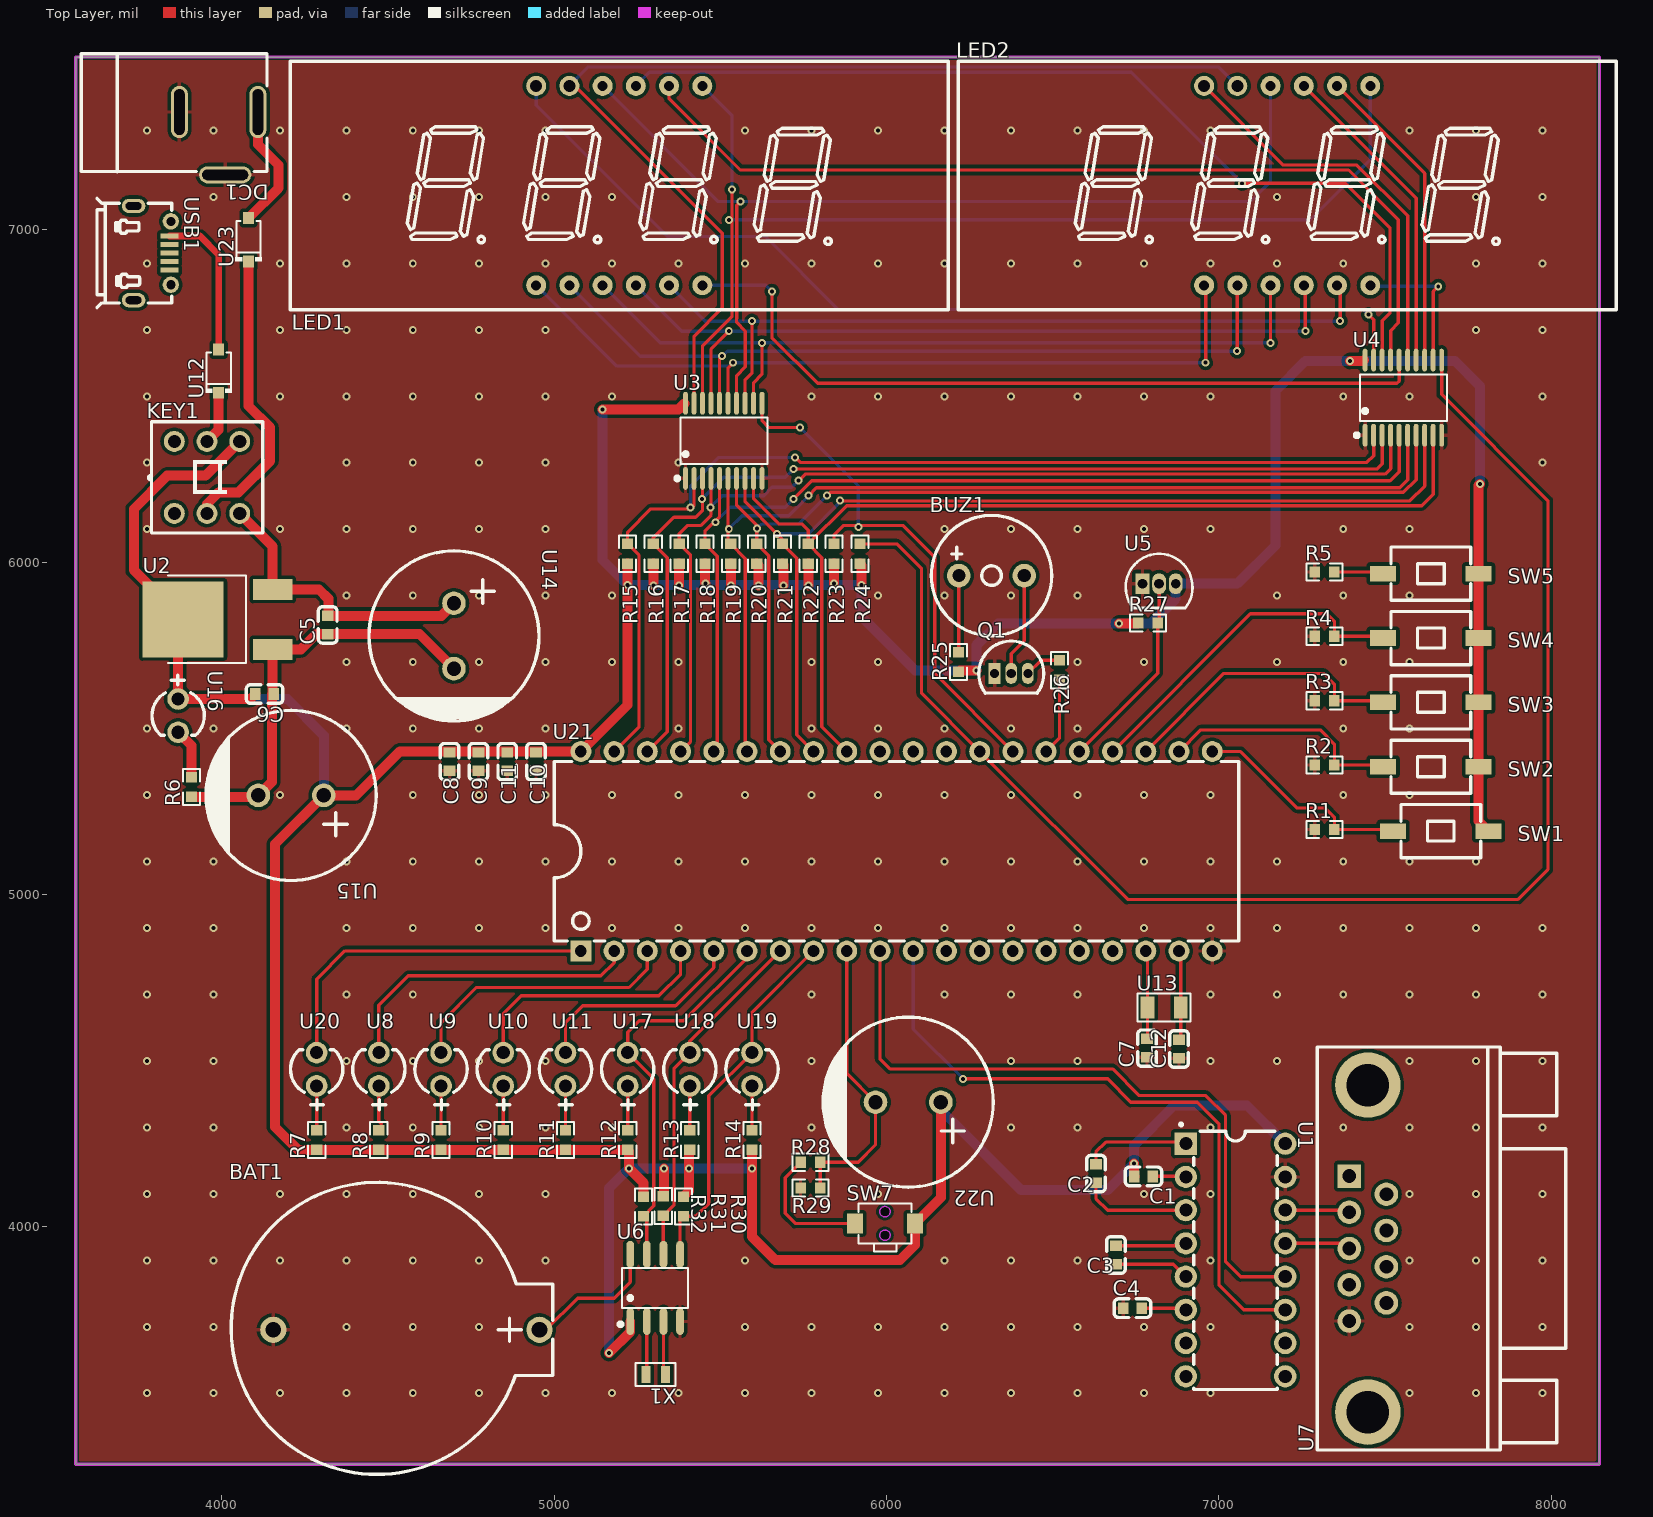
[diagram p0: Top Layer view]
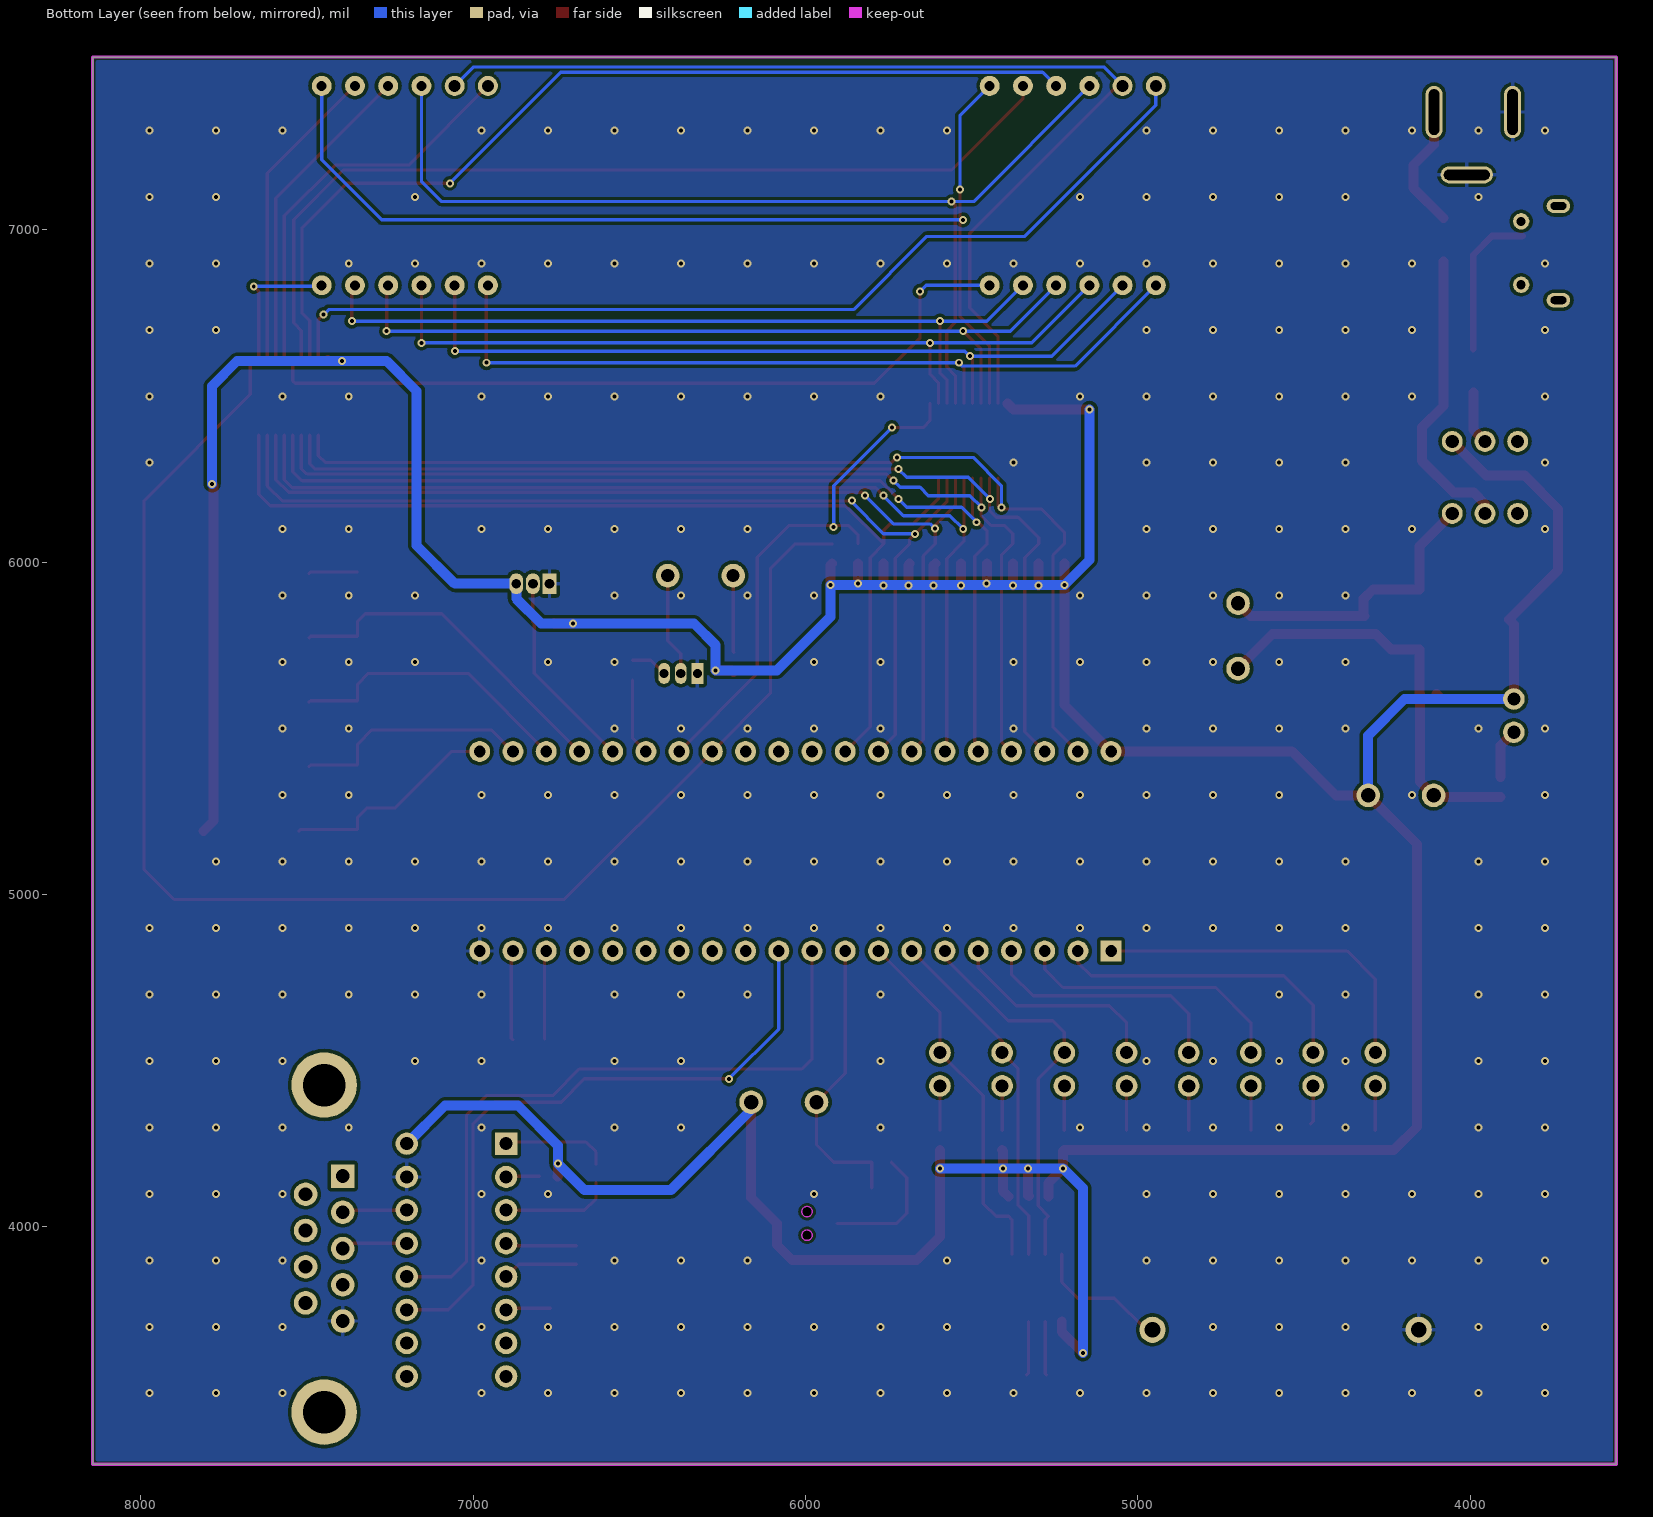
[diagram p1: Bottom Layer view, seen from below]
# Altium PCB MISC51895.pcbdoc
Units mil, origin at the board's own origin, x right, y up, seen from the top; angles counter-clockwise.
Board outline 4585 x 4235 mil, 2 copper layers (Top Layer, Bottom Layer), stack 62.206 mil thick; 82 components, 78 nets, 302 pads, 351 vias.

## Layer stack, top to bottom
Top Solder Mask Layer: solder mask 0.394, Dk 3.3
Top Layer: signal copper 1.379
Dielectric1: surface 59.449, FR4, Dk 4.5
Bottom Layer: signal copper 1.378
Bottom Solder Mask Layer: solder mask 0.394, Dk 3.3

## Board outline
3560,7520 3560,3285 8145,3285 8145,7520

## Design rules (kind name [scope] priority, off if disabled: settings)
BoardOutlineClearance copperThickness2oz_1 [All] p2 off: genericclearance=7.99 ignorepadtopadclearanceinfootprint=FALSE except(0: Arc-SplitContinuation Track-SplitContinuation SMDPad-SplitContinuation THPad-SplitContinuation Via-SplitContinuation Fill-SplitContinuation Region-SplitContinuation Poly-SplitContinuation Text-SplitContinuation Hole-SplitContinuation; 5.98: Arc-CutoutEdge SMDPad-CutoutEdge THPad-CutoutEdge Via-CutoutEdge Fill-CutoutEdge Region-CutoutEdge Text-CutoutEdge; 6.93: Hole-OutlineEdge Hole-CutoutEdge; 10: Poly-OutlineEdge Poly-CutoutEdge; 11.81: Arc-OutlineEdge Track-OutlineEdge SMDPad-OutlineEdge THPad-OutlineEdge Via-OutlineEdge Fill-OutlineEdge Region-OutlineEdge Text-OutlineEdge Track-CutoutEdge)
BoardOutlineClearance copperThickness1oz_1 [All] p4: genericclearance=4.02 ignorepadtopadclearanceinfootprint=FALSE except(0: Arc-SplitContinuation Track-SplitContinuation SMDPad-SplitContinuation THPad-SplitContinuation Via-SplitContinuation Fill-SplitContinuation Region-SplitContinuation Poly-SplitContinuation Text-SplitContinuation Hole-SplitContinuation; 6: SMDPad-CutoutEdge THPad-CutoutEdge Via-CutoutEdge Fill-CutoutEdge Region-CutoutEdge Text-CutoutEdge; 6.93: Hole-OutlineEdge Hole-CutoutEdge; 10: Poly-OutlineEdge Poly-CutoutEdge; 11.8: Arc-OutlineEdge Track-OutlineEdge SMDPad-OutlineEdge THPad-OutlineEdge Via-OutlineEdge Fill-OutlineEdge Region-OutlineEdge Text-OutlineEdge; 11.81: Arc-CutoutEdge Track-CutoutEdge)
Clearance copperThickness2oz [All] p1 off: gap=7.99 ignorepadtopadclearanceinfootprint=FALSE except(5.98: SMDPad-Track SMDPad-SMDPad THPad-Track SMDPad-THPad THPad-THPad Track-Via SMDPad-Via THPad-Via Via-Via Fill-Track Region-Track Fill-SMDPad Region-SMDPad Fill-THPad Region-THPad Fill-Via Region-Via Fill-Fill Fill-Region Region-Region Arc-Track Arc-SMDPad Arc-THPad Arc-Via Fill-Arc Region-Arc Arc-Arc Text-Track SMDPad-Text Text-THPad Text-Via Fill-Text Region-Text Arc-Text Text-Text; 6.93: Hole-Track Hole-SMDPad Hole-THPad Hole-Via Fill-Hole Region-Hole Hole-Arc Hole-Text; 10: Poly-Track Poly-SMDPad Poly-THPad Poly-Via Poly-Fill Poly-Region Poly-Poly Poly-Arc Poly-Text Poly-Hole)
Clearance copperThickness1oz [All] p3: gap=4.02 ignorepadtopadclearanceinfootprint=FALSE except(5.98: SMDPad-Track SMDPad-SMDPad THPad-Track SMDPad-THPad THPad-THPad Track-Via SMDPad-Via THPad-Via Via-Via Fill-Track Region-Track Fill-SMDPad Region-SMDPad Fill-THPad Region-THPad Fill-Via Region-Via Fill-Fill Fill-Region Region-Region; 6: Arc-Track Arc-SMDPad Arc-THPad Arc-Via Fill-Arc Region-Arc Arc-Arc Text-Track SMDPad-Text Text-THPad Text-Via Fill-Text Region-Text Arc-Text Text-Text; 6.93: Hole-Track Hole-SMDPad Hole-THPad Hole-Via Fill-Hole Region-Hole Hole-Arc Hole-Text; 10: Poly-Track Poly-SMDPad Poly-THPad Poly-Via Poly-Fill Poly-Region Poly-Poly Poly-Arc Poly-Text Poly-Hole)
DiffPairsRouting differentialPair [All] p1: maxlimit=6 minlimit=6 mostfreqgap=6 toplayer_minwidth=5 toplayer_prefwidth=10 toplayer_maxwidth=100 toplayer_mingap=6 toplayer_prefgap=6 toplayer_maxgap=6 bottomlayer_minwidth=5 bottomlayer_prefwidth=10 bottomlayer_maxwidth=100 bottomlayer_mingap=6 bottomlayer_prefgap=6 bottomlayer_maxgap=6 maxuncoupledlength=10
HoleToHoleClearance otherClearance [All] p1: gap=11.81 allowstackedmicrovias=TRUE
Length netLength [All] p1: minlimit=0 maxlimit=0
MatchedLengths netLengthTolerance [All] p1: tolerance=1000
PasteMaskExpansion pasteMaskExpansion [All] p1: expansion=0
PlaneConnect innerPlane [All] p1: planeconnectstyle=Relief reliefexpansion=20 reliefentries=4 reliefconductorwidth=10 reliefairgap=10
PolygonConnect copperRegion [(InNet('GND'))] p1: connectstyle=Relief reliefconductorwidth=10 reliefentries=4 polygonreliefangle="90 Angle" airgapwidth=10 via.connectstyle=Relief via.reliefconductorwidth=10 via.reliefentries=4 via.polygonreliefangle="90 Angle" via.airgapwidth=10
RoutingVias viaSize [All] p1: holewidth=12.01 width=24.02 viastyle="Through Hole" minholewidth=11.81 minwidth=19.68 maxholewidth=248.03 maxwidth=393.7
SolderMaskExpansion solderMaskExpansion [IsVia] p1: expansion=-1000 istentingtop=TRUE
SolderMaskExpansion solderMaskExpansion [All] p2: expansion=2 istentingtop=FALSE
Width copperThickness2oz_2 [All] p1 off: maxlimit=100 minlimit=8 preferedwidth=10
Width copperThickness1oz_2 [All] p2: maxlimit=100 minlimit=5 preferedwidth=10

## Components (designator, comment, footprint, x,y, rotation, side; value= is the part's Value field where it differs from the comment)
BAT1 "CR2032-2-1" BAT-TH_CR2032-2-1 4555,3690 r0 top
BUZ1 "Buzzer" BUZ-TH_BD9.0-P5.00-D0.6-FD 6315.73,5959.5 r0 top
C1 "104" C0603 6772.91,4151.65 r180 top
C2 "4.7uF" C0603 6630,4160 r90 top
C3 "4.7uF" C0603 6690,3915 r90 top
C4 "4.7uF" C0603 6740,3755 r0 top
C5 "4.7uF" C0603 4318.1,5811.04 r90 top
C6 "4.7uF" C0603 4128.22,5603.04 r180 top
C7 "100nF" C0603 6783.76,4537.58 r90 top
C8 "4.7uF" C0603 4685,5399.61 r90 top
C9 "4.7uF" C0603 4771.67,5399.61 r90 top
C10 "4.7uF" C0603 4945,5399.61 r90 top
C11 "4.7uF" C0603 4858.33,5399.61 r90 top
C12 "100nF" C0603 6880,4535 r90 top
DC1 "" DC-2.0 3985,7365 r180 top
KEY1 "Non-latching switch 8.5×8.5 silent" SW-TH_6P-L8.5-W8.5-P2.54 3955,6255 r0 top
LED1 "FJ5461AB" LED-SEG-TH_12P-L50.4-W19.0-P2.54-S15.24-BL 5195.44,7133.14 r0 top
LED2 "FJ5461AB" LED-SEG-TH_12P-L50.4-W19.0-P2.54-S15.24-BL 7205.45,7133.14 r0 top
Q1 "2SC945" TO-92-3_L4.9-W3.7-P1.27-L 6375,5665 r0 top
R1 "48.7Ω" R0603 7317.91,5195.61 r0 top
R2 "48.7Ω" R0603 7317.91,5389.3 r0 top
R3 "48.7Ω" R0603 7317.91,5583 r0 top
R4 "48.7Ω" R0603 7317.91,5776.69 r0 top
R5 "48.7Ω" R0603 7317.91,5970.38 r0 top
R6 "10K" R0603 3908.1,5323.04 r90 top
R7 "10K" R0603 4284.92,4261.14 r90 top
R8 "10K" R0603 4472.09,4261.14 r90 top
R9 "10K" R0603 4659.25,4261.14 r90 top
R10 "10K" R0603 4846.42,4261.14 r90 top
R11 "10K" R0603 5033.58,4261.14 r90 top
R12 "10K" R0603 5220.75,4261.14 r90 top
R13 "10K" R0603 5407.91,4261.14 r90 top
R14 "10K" R0603 5595.08,4261.14 r90 top
R15 "10K" R0603 5220.35,6025 r90 top
R16 "10K" R0603 5298.05,6025 r90 top
R17 "10K" R0603 5375.75,6025 r90 top
R18 "10K" R0603 5453.45,6025 r90 top
R19 "10K" R0603 5531.15,6025 r90 top
R20 "10K" R0603 5608.85,6025 r90 top
R21 "10K" R0603 5686.55,6025 r90 top
R22 "10K" R0603 5764.25,6025 r90 top
R23 "10K" R0603 5841.95,6025 r90 top
R24 "10K" R0603 5919.65,6025 r90 top
R25 "50" R0603 6216.06,5699.16 r90 top
R26 "1K" R0603 6520,5675 r90 top
R27 "10K" R0603 6786.25,5816.95 r0 top
R28 "10K" R0603 5770.79,4194.3 r180 top
R29 "10K" R0603 5770.79,4116.6 r0 top
R30 "4.7K" R0603 5388.55,4061.02 r270 top
R31 "4.7K" R0603 5327.76,4062.64 r270 top
R32 "4.7K" R0603 5268.55,4061.02 r270 top
SW1 "SW_PB_ESW_1" KEY-SMD_L6.1-W3.8-LS8.0 7667.63,5190.61 r0 top
SW2 "SW_PB_ESW_1" KEY-SMD_L6.1-W3.8-LS8.0 7637.63,5384.3 r0 top
SW3 "SW_PB_ESW_1" KEY-SMD_L6.1-W3.8-LS8.0 7637.63,5578 r0 top
SW4 "SW_PB_ESW_1" KEY-SMD_L6.1-W3.8-LS8.0 7637.63,5771.69 r0 top
SW5 "SW_PB_ESW_1" KEY-SMD_L6.1-W3.8-LS8.0 7637.63,5965.38 r0 top
SW7 "YD-3410" SW-SMD_L3.9-W2.9-LS4.8-EH-A 5995,4010 r0 top
U1 "MAX232AEJE" PDIP-16_L19.3-W6.5-P2.54-LS7.6-BL 7050,3900 r270 top
U2 "LM1117IDT-5.0" TO-252-2_L6.6-W6.1-P4.57-LS9.7-BR-CW 4017.9,5827.5 r0 top
U3 "74HC573PW/AU118" TSSOP-20_L6.5-W4.4-P0.65-LS6.4-BL 5510,6365 r0 top
U4 "74HC573PW/AU118" TSSOP-20_L6.5-W4.4-P0.65-LS6.4-BL 7555,6495 r0 top
U5 "DS18B20+T&R-HX" TO-92-3_L5.1-W4.1-P1.27-L-1 6820,5935 r0 top
U6 "DS1302Z+T&R-TUDI" SOIC-8_L4.9-W3.9-P1.27-LS6.0-BL 5303.55,3816.02 r0 top
U7 "DB9F" DB9-TH_DB9F_C9900018961 7448.11,3934.4 r90 top
U8 "LED" LED-TH_BD4.0-P2.54-FD_RED 4472.09,4473.89 r90 top
U9 "LED" LED-TH_BD4.0-P2.54-FD_RED 4659.25,4473.89 r90 top
U10 "LED" LED-TH_BD4.0-P2.54-FD_RED 4846.42,4473.89 r90 top
U11 "LED" LED-TH_BD4.0-P2.54-FD_RED 5033.58,4473.89 r90 top
U12 "IN5819" SOD-123_L2.7-W1.7-LS3.8-RD 3990,6575 r90 top
U13 "2.768KHz" CRYSTAL-SMD_L3.2-W1.5-1 6835,4660 r0 top
U14 "CE63V1000uF13*25" CAP-TH_BD13.0-P5.00-D0.6-FD 4698.1,5778.04 r270 top
U15 "10uF" CAP-TH_BD13.0-P5.00-D0.6-FD 4208.1,5298.04 r180 top
U16 "LED" LED-TH_BD4.0-P2.54-FD_RED 3868.1,5538.04 r270 top
U17 "LED" LED-TH_BD4.0-P2.54-FD_RED 5220.75,4473.89 r90 top
U18 "LED" LED-TH_BD4.0-P2.54-FD_RED 5407.91,4473.89 r90 top
U19 "LED" LED-TH_BD4.0-P2.54-FD_RED 5595.08,4473.89 r90 top
U20 "LED" LED-TH_BD4.0-P2.54-FD_RED 4284.92,4473.89 r90 top
U21 "STC89C53RC-40I-PDIP40" DIP-40_L52.0-W13.7-P2.54-LS15.2-BL 6030,5130 r0 top
U22 "CE63V1000uF13*25" CAP-TH_BD13.0-P5.00-D0.6-FD 6065,4375 r180 top
U23 "IN5819" SOD-123_L2.7-W1.7-LS3.8-RD 4080,6970 r90 top
USB1 "MICRO-USB-1" MICRO-USB-SMD_C9900008946 3790,6930 r270 top
X1 "32.768K" OSC-SMD_L2.0-W1.2 5305,3555 r180 top

## Footprints (in the part's own frame and the unit in brackets; to place one, negate y for a bottom-side part, rotate by r counter-clockwise, add the part's x,y. Pads: shape width x height; smd on the part's side, far side on the other; paste and mask are expansions set on the pad)
BAT-TH_CR2032-2-1 [mm]
  round 2 hole 1.2: 1(10.175,0) 2(-10.175,0)
  silkscreen extent -13.4,-11.05 11.17,11.26
BUZ-TH_BD9.0-P5.00-D0.6-FD [mm]
  round 1.8 hole 1 copper offset 0,0: 1(-2.5,0)
  round 1.8 hole 1: 2(2.5,0)
  silkscreen extent -4.6,-4.6 4.6,4.6
C0603 [mm]
  rect 0.8x0.9 smd: 1(-0.7,0) 2(0.7,0)
  silkscreen extent -1.39,-0.71 1.39,0.71
CAP-TH_BD13.0-P5.00-D0.6-FD [mm]
  round 1.8 hole 1.1: 1(-2.5,0) 2(2.5,0)
  silkscreen extent -6.5,-6.5 6.5,6.5
CRYSTAL-SMD_L3.2-W1.5-1 [mm]
  rect 1.05x1.7 smd: 1(-1.275,0) 2(1.275,0)
  silkscreen extent -2.03,-1.08 2.03,1.08
DB9-TH_DB9F_C9900018961 [mm]
  rect 1.8x1.8 hole 1.05 paste+0 mask+0.05: 1(5.54,1.42)
  round 1.8 hole 1.05 paste+0 mask+0.05: 2(2.77,1.42) 3(0,1.42) 4(-2.77,1.42) 5(-5.54,1.42) 6(4.155,-1.42) 7(1.385,-1.42) 8(-1.385,-1.42) 9(-4.155,-1.42)
  round 5 hole 3.25 paste+0 mask+0.05: 10(-12.5,0) 11(12.5,0)
  silkscreen extent -15.4,-15.13 15.4,3.87
DC-2.0 [mil]
  oval 157.5x51.2 hole 31.5 slot 137.8 at 0 deg paste+0 mask+2: 2(-24.7,199.5)
  oval 51.2x157.5 hole 31.5 slot 137.8 at 90 deg paste+0 mask+2: 3(113.1,10.5) 4(-123.1,10.5)
  silkscreen extent -151,-165 408,190
DIP-40_L52.0-W13.7-P2.54-LS15.2-BL [mil]
  rect 63x63 hole 35: 1(-950,-300)
  round 63 hole 35: 2(-850,-300) 3(-750,-300) 4(-650,-300) 5(-550,-300) 6(-450,-300) 7(-350,-300) 8(-250,-300) 9(-150,-300) 10(-50,-300) 11(50,-300) 12(150,-300) 13(250,-300) 14(350,-300) 15(450,-300) 16(550,-300) 17(650,-300) 18(750,-300) 19(850,-300) 20(950,-300) 21(950,300) 22(850,300) 23(750,300) 24(650,300) 25(550,300) 26(450,300) 27(350,300) 28(250,300) 29(150,300) 30(50,300) 31(-50,300) 32(-150,300) 33(-250,300) 34(-350,300) 35(-450,300) 36(-550,300) 37(-650,300) 38(-750,300) 39(-850,300) 40(-950,300)
  silkscreen extent -1030,-270 1030,270
KEY-SMD_L6.1-W3.8-LS8.0 [mm]
  rect 2x1.2 smd: 1(-3.65,0) 2(3.65,0)
  silkscreen extent -3.05,-2.03 3.05,2.03
LED-SEG-TH_12P-L50.4-W19.0-P2.54-S15.24-BL [mil]
  round 60 hole 30: 1(-250,-300) 2(-150,-300) 3(-50,-300) 4(50,-300) 5(150,-300) 6(250,-300) 7(250,300) 8(150,300) 9(50,300) 10(-50,300)
  round 60 hole 36: 11(-150,300) 12(-250,300)
  silkscreen extent -990,-374 990,374
LED-TH_BD4.0-P2.54-FD_RED [mil]
  round 65 hole 39.37: 1(-50,0) 2(50,0)
  silkscreen extent -122,-79 59,79
MICRO-USB-SMD_C9900008946 [mm]
  rect 0.4x1.35 smd paste-100 mask+0.051: 1(-1.3,1.325) 2(-0.65,1.325) 3(0,1.325) 4(0.65,1.325) 5(1.3,1.325)
  oval 1.1x1.8 hole 0.6 slot 1.2 at 90 deg: 6(-3.6,-1.425) 6(3.6,-1.425)
  round 1.25 hole 0.7: 6(-2.425,1.425) 6(2.425,1.425)
  silkscreen extent -4.19,-4.22 4.19,1.5
OSC-SMD_L2.0-W1.2 [mm]
  rect 0.7x1.3 smd: 1(-0.75,0) 2(0.75,0)
  silkscreen extent -1.53,-0.88 1.53,0.88
PDIP-16_L19.3-W6.5-P2.54-LS7.6-BL [mm]
  rect 1.7x1.7 hole 1: 1(-8.89,-3.8)
  round 1.7 hole 1: 2(-6.35,-3.8) 3(-3.81,-3.8) 4(-1.27,-3.8) 5(1.27,-3.8) 6(3.81,-3.8) 7(6.35,-3.8) 8(8.89,-3.8) 9(8.89,3.8) 10(6.35,3.8) 11(3.81,3.8) 12(1.27,3.8) 13(-1.27,3.8) 14(-3.81,3.8) 15(-6.35,3.8) 16(-8.89,3.8)
  silkscreen extent -10.46,-4.26 9.9,3.2
R0603 [mil]
  rect 31.75x34.02 smd paste-3937.01 mask+2: 1(-29.66,0) 2(29.66,0)
  silkscreen extent -55,-26 55,26
SOD-123_L2.7-W1.7-LS3.8-RD [mm]
  rect 0.91x0.84 smd: 1(-1.655,0) 2(1.655,0)
  silkscreen extent -1.65,-1 1.43,1
SOIC-8_L4.9-W3.9-P1.27-LS6.0-BL [mm]
  oval 0.588x2.045 smd: 1(-1.905,-2.57) 2(-0.635,-2.57) 3(0.635,-2.57) 4(1.905,-2.57) 5(1.905,2.57) 6(0.635,2.57) 7(-0.635,2.57) 8(-1.905,2.57)
  silkscreen extent -2.8,-2.92 2.53,1.52
SW-SMD_L3.9-W2.9-LS4.8-EH-A [mm]
  rect 1.23x1.5 smd: 1(-2.3,0) 2(2.3,0)
  Board Outline Layer circle w0.003: c0,-0.9 r0.4
  Board Outline Layer circle w0.003: c0,0.9 r0.4
  Board Outline Layer region: 0.4,-0.9 0.36,-1.073 0.249,-1.213 0.089,-1.29 -0.089,-1.29 -0.249,-1.213 -0.36,-1.073 -0.4,-0.9 -0.4,-0.9 -0.36,-0.726 -0.249,-0.587 -0.089,-0.51 0.089,-0.51 0.249,-0.587 0.36,-0.726 0.4,-0.9
  Board Outline Layer region: 0.4,-0.9 0.39,-0.989 0.36,-1.073 0.313,-1.149 0.249,-1.213 0.174,-1.26 0.089,-1.29 0,-1.3 -0.089,-1.29 -0.174,-1.26 -0.249,-1.213 -0.313,-1.149 -0.36,-1.073 -0.39,-0.989 -0.4,-0.9 -0.39,-0.811 -0.36,-0.726 -0.313,-0.65 -0.249,-0.587 -0.174,-0.539 -0.089,-0.51 0,-0.5 0.089,-0.51 0.174,-0.539 0.249,-0.587 0.313,-0.65 0.36,-0.726 0.39,-0.811
  Board Outline Layer region: 0.4,0.9 0.36,0.726 0.249,0.587 0.089,0.51 -0.089,0.51 -0.249,0.587 -0.36,0.726 -0.4,0.9 -0.4,0.9 -0.36,1.074 -0.249,1.213 -0.089,1.29 0.089,1.29 0.249,1.213 0.36,1.074 0.4,0.9
  Board Outline Layer region: 0.4,0.9 0.39,0.811 0.36,0.726 0.313,0.651 0.249,0.587 0.174,0.54 0.089,0.51 0,0.5 -0.089,0.51 -0.174,0.54 -0.249,0.587 -0.313,0.651 -0.36,0.726 -0.39,0.811 -0.4,0.9 -0.39,0.989 -0.36,1.074 -0.313,1.149 -0.249,1.213 -0.174,1.26 -0.089,1.29 0,1.3 0.089,1.29 0.174,1.26 0.249,1.213 0.313,1.149 0.36,1.074 0.39,0.989
  Multi-Layer board cut-out: 0.4,-0.9 0.36,-1.073 0.249,-1.213 0.089,-1.29 -0.089,-1.29 -0.249,-1.213 -0.36,-1.073 -0.4,-0.9 -0.4,-0.9 -0.36,-0.726 -0.249,-0.587 -0.089,-0.51 0.089,-0.51 0.249,-0.587 0.36,-0.726 0.4,-0.9
  Multi-Layer board cut-out: 0.4,0.9 0.36,0.726 0.249,0.587 0.089,0.51 -0.089,0.51 -0.249,0.587 -0.36,0.726 -0.4,0.9 -0.4,0.9 -0.36,1.074 -0.249,1.213 -0.089,1.29 0.089,1.29 0.249,1.213 0.36,1.074 0.4,0.9
  silkscreen extent -2.03,-2.16 2.03,1.54
SW-TH_6P-L8.5-W8.5-P2.54 [mm]
  round 1.6 hole 1: 1(-2.5,-2.75) 2(0,-2.75) 3(2.5,-2.75) 4(-2.5,2.75) 5(0,2.75) 6(2.5,2.75)
  silkscreen extent -4.47,-4.25 4.25,4.25
TO-92-3_L4.9-W3.7-P1.27-L [mm]
  rect 0.9x1.6 hole 0.7: 1(-1.27,0)
  oval 0.9x1.6 hole 0.7: 2(0,0) 3(1.27,0)
  silkscreen extent -2.48,-1.5 2.48,2.48
TO-92-3_L5.1-W4.1-P1.27-L-1 [mm]
  rect 1.05x1.6 hole 0.75: 1(-1.27,0)
  oval 1.05x1.6 hole 0.75: 2(0,0) 3(1.27,0)
  silkscreen extent -2.55,-1.87 2.55,2.29
TO-252-2_L6.6-W6.1-P4.57-LS9.7-BR-CW [mm]
  rect 3x1.6 smd: 1(3.424,-2.29) 3(3.424,2.29)
  rect 6.2x5.8 smd: 2(-3.424,0)
  silkscreen extent -4.58,-3.35 1.38,3.35
TSSOP-20_L6.5-W4.4-P0.65-LS6.4-BL [mil]
  oval 14.33x68.58 smd: 1(-115.16,-113.03) 2(-89.57,-113.03) 3(-63.98,-113.03) 4(-38.39,-113.03) 5(-12.79,-113.03) 6(12.8,-113.03) 7(38.39,-113.03) 8(63.98,-113.03) 9(89.57,-113.03) 10(115.16,-113.03) 11(115.16,113.03) 12(89.57,113.03) 13(63.98,113.03) 14(38.39,113.03) 15(12.8,113.03) 16(-12.79,113.03) 17(-38.39,113.03) 18(-63.98,113.03) 19(-89.57,113.03) 20(-115.16,113.03)
  silkscreen extent -146,-119 131,70

## Via types
v1: diameter 24.02, hole 12, Top Layer to Bottom Layer, 351 vias

## Nets (pads, with @x,y where several pads share a name; then routed paths per layer and width w, separated by ;. In a path a pad name is that pad's centre, name@x,y a point inside that pad or via, vN(x,y) a via of type N, cw(c..) or ccw(c..) an arc to the next point about the centre after c; other vN are vias at no path point)
$1N44: U12.2 USB1.1 | length 455.9
  Top Layer w20: USB1.1 3933.82,6981.18 3990,6925 U12.2
$1N57: C4.2 U1.6 | length 134.9
  Top Layer w10: C4.2 6895.39,3755 U1.6
$1N71: C2.2 U1.1 | length 322.3
  Top Layer w10: C2.2 6630,4225 6660,4255 6895.39,4255 U1.1
$1N83: U1.13 U7.3 | length 199
  Top Layer w10: U1.13 7376.61,3950 U7.3
$1N85: U1.14 U7.2 | length 195.3
  Top Layer w10: U1.14 7385.66,4050 U7.2
$1N94: C5.1 C6.1 R6.1 U2.1 U14.2 U15.2 | length 1268.2
  Top Layer w30: R6.1 4105.01,5293.38 U15.2 4150.54,5338.91 4150.54,5603.04 4152.7,5605.2 U2.1 4237.34,5737.34 4283.48,5783.48 C5.1 4594.23,5783.48 U14.2
$1N97: R6.2 U16.2 | length 151.9
  Top Layer w30: U16.2 3908.1,5448.04 R6.2
$1N98: R7.2 U20.1 | length 133.1
  Top Layer w10: R7.2 U20.1
$1N99: R8.2 U8.1 | length 117.2
  Top Layer w10: U8.1 4472.09,4317.91 4480,4310
$1N101: R9.2 U9.1 | length 133.1
  Top Layer w10: R9.2 U9.1
$1N102: R10.2 U10.1 | length 133.1
  Top Layer w10: R10.2 U10.1
$1N103: R11.2 U11.1 | length 133.1
  Top Layer w10: R11.2 U11.1
$1N104: R12.2 U17.1 | length 133.1
  Top Layer w10: R12.2 U17.1
$1N105: R13.2 U18.1 | length 133.1
  Top Layer w10: R13.2 U18.1
$1N106: R14.2 U19.1 | length 133.1
  Top Layer w10: R14.2 U19.1
$1N124: BUZ1.2 Q1.2 | length 310.7
  Top Layer w10: Q1.2 6375,5725 6414.15,5764.15 BUZ1.2@6414.15,5959.5
$1N125: BUZ1.1 R25.2 | length 231.2
  Top Layer w10: R25.2 6217.3,5730.07 BUZ1.1
$1N126: Q1.3 R26.2 | length 111.4
  Top Layer w10: Q1.3 6464.66,5704.66 R26.2
$1N142: R28.2 SW7.1 | length 395.3
  Top Layer w10: R28.2 5695,4148.18 5695,4040 5725,4010 SW7.1
$1N143: R28.1 R29.2 U21.9 U22.2 | length 884.8
  Top Layer w10: R29.2 R28.1 5914.3,4194.3 5966.57,4246.57 U22.2 5880,4461.57 U21.9
$1N146: C12.2 U13.2 U21.19 | length 271.7
  Top Layer w10: C12.2 6885.19,4567.75 U13.2 6885.19,4824.81 U21.19
$1N148: C7.2 U13.1 U21.18 | length 267.3
  Top Layer w10: U21.18 6784.8,4825.2 U13.1 6784.8,4566.18 C7.2
$1N151: C1.1 U1.2 | length 100.6
  Top Layer w10: C1.1 6898.74,4151.65 U1.2
$1N153: C2.1 U1.3 | length 332.3
  Top Layer w10: C2.1 6630,4085 6665,4050 U1.3
$1N155: C3.1 U1.5 | length 225.9
  Top Layer w10: C3.1 6862.95,3887.44 U1.5
$1N156: C3.2 U1.4 | length 213.5
  Top Layer w10: C3.2 6892.95,3942.56 U1.4
$1N167: U6.2 X1.2 | length 161.1
  Top Layer w10: X1.2 5278.55,3558.07 U6.2
$1N168: U6.3 X1.1 | length 162.3
  Top Layer w10: U6.3 5328.55,3560.98 X1.1
$1N170: BAT1.1 U6.8 | length 416.1
  Top Layer w10: BAT1.1 4975,3690 5070,3785 5180,3785 5228.55,3833.55 U6.8
$1N260: KEY1.5 U12.1 | length 161.1
  Top Layer w30: KEY1.5 3990,6398.27 U12.1
$1N266: DC1.4 U23.2 | length 382.3
  Top Layer w30: U23.2 4170,7125.16 4170,7195 4108.1,7256.9 DC1.4
+5V: C1.2 C6.2 C8.2 C9.2 C10.2 C11.2 KEY1.6 R7.1 R8.1 R9.1 R10.1 R11.1 R12.1 R13.1 R14.1 R15.1 R16.1 R17.1 R18.1 R19.1 R20.1 R21.1 R22.1 R23.1 R24.1 R25.1 R27.1 R30.1 R31.1 R32.1 SW1.2 SW2.2 SW3.2 SW4.2 SW5.2 SW7.2 U1.16 U2.2 U3.20 U4.20 U5.3 U6.1 U15.1 U16.1 U21.40 U22.1 | length 16051.5
  Top Layer w30: KEY1.6 3950.16,6260 3835,6260 3735,6160 3735,5975.59 U2.2 3868.1,5812.5 U16.1 4085.66,5588.04 C6.2 ; v1(5145,6460) 5374.25,6460 U3.20@5392.28,6478.03 ; v1(5165,3620) 5228.55,3683.55 U6.1 ; R15.1 v1(5220.35,5931.52) 5220.35,5570.35 U21.40 4535,5430 4403.04,5298.04 U15.1 4160,5151.52 4160,4300 4228.52,4231.48 R7.1 R8.1 R9.1 R10.1 R11.1 R12.1 5225,4227.23 v1(5225,4176) 5268.55,4132.45 R32.1 ; v1(5298.05,5930) R16.1 ; R31.1 5330,4094.53 v1(5330,4176) ; v1(5375.75,5930) R17.1 ; R30.1 5405,4107.14 v1(5405,4176) 5405,4228.57 R13.1 ; R18.1 5453.45,5936.55 v1(5455,5935) ; v1(5531.15,5930) R19.1 ; R14.1 v1(5595.08,4176) 5595.08,3969.92 5665,3900 6040,3900 6085.55,3945.55 SW7.2 6163.43,4087.88 U22.1 ; R20.1 5615,5989.19 v1(5615,5930) ; R21.1 5690,5991.89 v1(5690,5930) ; R22.1 5765,5994.59 v1(5765,5930) ; v1(5841.95,5935) R23.1 ; R24.1 5925,5989.99 v1(5925,5931.52) ; R25.1 6221.06,5674.5 v1(6270,5674.5) ; v1(6700,5815) 6754.64,5815 R27.1 ; v1(6745,4190) 6745,4152.01 C1.2 ; v1(7395,6605) 7434.25,6605 U4.20@7437.28,6608.03 ; v1(7785,6235) 7781.33,6231.33 SW5.2 SW4.2 SW3.2 SW2.2 7781.33,5220.61 SW1.2
  Bottom Layer w30: U16.1 4196.96,5588.04 4306.52,5478.48 U15.1 ; v1(5145,6460) 5145,6006.86 v1(5220.35,5931.52) v1(5925,5931.52) 5925,5835 6085.5,5674.5 v1(6270,5674.5) 6270,5750 6335,5815 v1(6700,5815) 6795,5815 6870,5890 U5.3 7055,5935 7170,6050 7170,6515 7260,6605 v1(7395,6605) 7710,6605 7785,6530 v1(7785,6235) ; v1(5165,3620) 5165,4116 v1(5225,4176) v1(5330,4176) v1(5405,4176) v1(5595.08,4176) ; U22.1 6163.43,4351.57 6405,4110 6665,4110 v1(6745,4190) 6745,4245 6865,4365 7084.61,4365 U1.16
+9V: C5.2 KEY1.3 U2.3 U14.1 | length 896.8
  Top Layer w30: KEY1.3 4152.7,6047.46 U2.3 4292.34,5917.66 4320,5890 4320,5840.5 C5.2 4660.23,5838.6 U14.1
A: LED1.11 LED2.11 U3.19 | length 3247.2
  Top Layer w10: LED1.11 5061.86,7433.14 5505,6990 5505,6765 5420.43,6680.43 U3.19
  Bottom Layer w10: LED1.11 5102.3,7490 6998.58,7490 LED2.11
B: LED1.7 LED2.7 U3.18 | length 3255.9
  Top Layer w10: U3.18 5446.02,6651.02 5535,6740 v1(5535,7121.37)
  Bottom Layer w10: LED1.7 5535,7343.58 v1(5535,7121.37) ; v1(5526.02,7030) 7275,7030 7455.44,7210.44 LED2.7
C: LED1.4 LED2.4 U3.17 | length 2450.9
  Top Layer w10: U3.17 5471.61,6641.61 v1(5525,6695) ; LED2.4 7260,6828.58 v1(7260,6695)
  Bottom Layer w10: LED1.4 5383.58,6695 v1(5525,6695) v1(7260,6695)
D: LED1.2 LED2.2 U3.16 | length 2447.6
  Top Layer w10: U3.16 5497.21,6612.21 v1(5505,6620) ; v1(7055,6635) 7055,6832.69 LED2.2
  Bottom Layer w10: LED1.2 5258.58,6620 v1(5505,6620) 5520,6635 v1(7055,6635)
DP: LED1.3 LED2.3 U3.12 | length 2447.1
  Top Layer w10: U3.12 5599.57,6539.57 5625,6565 v1(5625,6660) ; v1(7155,6660) 7155,6832.69 LED2.3
  Bottom Layer w10: LED1.3 5318.58,6660 v1(5625,6660) v1(7155,6660)
E: LED1.1 LED2.1 U3.15 | length 2482.6
  Top Layer w10: U3.15 5522.8,6585 v1(5537.8,6600) ; LED2.1 6960,6828.58 v1(6960,6600)
  Bottom Layer w10: LED1.1 5188.58,6590 5527.8,6590 v1(5537.8,6600) v1(6960,6600)
F: LED1.10 LED2.10 U3.14 | length 3100.8
  Top Layer w10: U3.14 5548.39,6560.68 5575,6587.29 5575,6694.53 5548.39,6721.14 5548.39,6733.57 5549.02,6734.19 5549.02,7074.02 v1(5560,7085)
  Bottom Layer w10: LED1.10 5493.58,7085 v1(5560,7085) 7095,7085 7155.44,7145.44 LED2.10
G: LED1.5 LED2.5 U3.13 | length 2432.1
  Top Layer w10: U3.13 5573.98,6548.98 5595,6570 v1(5595,6725) ; LED2.5 7365,6823.58 v1(7365,6725)
  Bottom Layer w10: LED1.5 5453.58,6725 v1(5595,6725) v1(7365,6725)
GND: BAT1.2 C4.1 C7.1 C8.1 C9.1 C10.1 C11.1 C12.1 DC1.2 DC1.3 Q1.1 R1.1 R2.1 R3.1 R4.1 R5.1 R29.1 U1.15 U3.1 U3.10 U4.1 U4.10 U5.1 U6.4 U7.5 U21.20
  other v1: 3774.1,3499.1 3974.1,3499.1 4174.1,3499.1 4374.1,3499.1 4574.1,3499.1 4774.1,3499.1 4974.1,3499.1 5174.1,3499.1 5374.1,3499.1 5574.1,3499.1 5774.1,3499.1 5974.1,3499.1 6174.1,3499.1 6374.1,3499.1 6574.1,3499.1 6774.1,3499.1 6974.1,3499.1 7574.1,3499.1 7774.1,3499.1 7974.1,3499.1 3774.1,3699.1 3974.1,3699.1 4374.1,3699.1 4574.1,3699.1 4774.1,3699.1 5574.1,3699.1 5774.1,3699.1 5974.1,3699.1 6174.1,3699.1 6374.1,3699.1 6574.1,3699.1 6774.1,3699.1 6974.1,3699.1 7574.1,3699.1 7774.1,3699.1 7974.1,3699.1 3774.1,3899.1 3974.1,3899.1 4174.1,3899.1 4374.1,3899.1 4574.1,3899.1 4774.1,3899.1 4974.1,3899.1 5574.1,3899.1 6174.1,3899.1 6374.1,3899.1 6574.1,3899.1 6974.1,3899.1 7574.1,3899.1 7774.1,3899.1 7974.1,3899.1 3774.1,4099.1 3974.1,4099.1 4174.1,4099.1 4374.1,4099.1 4574.1,4099.1 4774.1,4099.1 4974.1,4099.1 5974.1,4099.1 6774.1,4099.1 6974.1,4099.1 7574.1,4099.1 7774.1,4099.1 7974.1,4099.1 3774.1,4299.1 3974.1,4299.1 4374.1,4299.1 4574.1,4299.1 4774.1,4299.1 4974.1,4299.1 5174.1,4299.1 5774.1,4299.1 6374.1,4299.1 6574.1,4299.1 6974.1,4299.1 7374.1,4299.1 7574.1,4299.1 7774.1,4299.1 7974.1,4299.1 3774.1,4499.1 3974.1,4499.1 4374.1,4499.1 4574.1,4499.1 4774.1,4499.1 4974.1,4499.1 5774.1,4499.1 6374.1,4499.1 6574.1,4499.1 6974.1,4499.1 7174.1,4499.1 7574.1,4499.1 7774.1,4499.1 7974.1,4499.1 3774.1,4699.1 3974.1,4699.1 4374.1,4699.1 4574.1,4699.1 5774.1,4699.1 6174.1,4699.1 6374.1,4699.1 6574.1,4699.1 6974.1,4699.1 7174.1,4699.1 7374.1,4699.1 7574.1,4699.1 7774.1,4699.1 7974.1,4699.1 3774.1,4899.1 3974.1,4899.1 4374.1,4899.1 4574.1,4899.1 4774.1,4899.1 4974.1,4899.1 5174.1,4899.1 5374.1,4899.1 5574.1,4899.1 5774.1,4899.1 5974.1,4899.1 6174.1,4899.1 6374.1,4899.1 6574.1,4899.1 6774.1,4899.1 6974.1,4899.1 7174.1,4899.1 7374.1,4899.1 7574.1,4899.1 7774.1,4899.1 7974.1,4899.1 3774.1,5099.1 3974.1,5099.1 4374.1,5099.1 4574.1,5099.1 4774.1,5099.1 4974.1,5099.1 5174.1,5099.1 5374.1,5099.1 5574.1,5099.1 5774.1,5099.1 5974.1,5099.1 6174.1,5099.1 6374.1,5099.1 6574.1,5099.1 6774.1,5099.1 6974.1,5099.1 7174.1,5099.1 7374.1,5099.1 7574.1,5099.1 7774.1,5099.1 3774.1,5299.1 4174.1,5299.1 4574.1,5299.1 4774.1,5299.1 4974.1,5299.1 5174.1,5299.1 5374.1,5299.1 5574.1,5299.1 5774.1,5299.1 5974.1,5299.1 6174.1,5299.1 6374.1,5299.1 6574.1,5299.1 6774.1,5299.1 6974.1,5299.1 7374.1,5299.1 7574.1,5299.1 3774.1,5499.1 3974.1,5499.1 4374.1,5499.1 4574.1,5499.1 4774.1,5499.1 4974.1,5499.1 5374.1,5499.1 5774.1,5499.1 5974.1,5499.1 6174.1,5499.1 6374.1,5499.1 6574.1,5499.1 7374.1,5499.1 7574.1,5499.1 4374.1,5699.1 4574.1,5699.1 4774.1,5699.1 4974.1,5699.1 5174.1,5699.1 5374.1,5699.1 5774.1,5699.1 5974.1,5699.1 6574.1,5699.1 6774.1,5699.1 7174.1,5699.1 7374.1,5699.1 7574.1,5699.1 4374.1,5899.1 4574.1,5899.1 4774.1,5899.1 4974.1,5899.1 5174.1,5899.1 5974.1,5899.1 6174.1,5899.1 6374.1,5899.1 6574.1,5899.1 7174.1,5899.1 7374.1,5899.1 7574.1,5899.1 3774.1,6099.1 4174.1,6099.1 4374.1,6099.1 4574.1,6099.1 4774.1,6099.1 4974.1,6099.1 6174.1,6099.1 6374.1,6099.1 6574.1,6099.1 6774.1,6099.1 6974.1,6099.1 7374.1,6099.1 7574.1,6099.1 3774.1,6299.1 4374.1,6299.1 4574.1,6299.1 4774.1,6299.1 4974.1,6299.1 5374.1,6299.1 7974.1,6299.1 3774.1,6499.1 4174.1,6499.1 4374.1,6499.1 4574.1,6499.1 4774.1,6499.1 4974.1,6499.1 5174.1,6499.1 5774.1,6499.1 5974.1,6499.1 6174.1,6499.1 6374.1,6499.1 6574.1,6499.1 6774.1,6499.1 6974.1,6499.1 7374.1,6499.1 7574.1,6499.1 7974.1,6499.1 3774.1,6699.1 4174.1,6699.1 4374.1,6699.1 4574.1,6699.1 4774.1,6699.1 4974.1,6699.1 7774.1,6699.1 7974.1,6699.1 3774.1,6899.1 4174.1,6899.1 4374.1,6899.1 4574.1,6899.1 4774.1,6899.1 4974.1,6899.1 5174.1,6899.1 5374.1,6899.1 5574.1,6899.1 5774.1,6899.1 5974.1,6899.1 6174.1,6899.1 6374.1,6899.1 6574.1,6899.1 6774.1,6899.1 6974.1,6899.1 7174.1,6899.1 7374.1,6899.1 7774.1,6899.1 7974.1,6899.1 3974.1,7099.1 4374.1,7099.1 4574.1,7099.1 4774.1,7099.1 4974.1,7099.1 5174.1,7099.1 7174.1,7099.1 7774.1,7099.1 7974.1,7099.1 3774.1,7299.1 3974.1,7299.1 4174.1,7299.1 4374.1,7299.1 4574.1,7299.1 4774.1,7299.1 4974.1,7299.1 5574.1,7299.1 5774.1,7299.1 5974.1,7299.1 6174.1,7299.1 6374.1,7299.1 6574.1,7299.1 6774.1,7299.1 6974.1,7299.1 7574.1,7299.1 7774.1,7299.1 7974.1,7299.1
K1: R1.2 SW1.1 U21.21 | length 664.7
  Top Layer w10: U21.21 7065,5430 7235,5260 7320,5260 7347.57,5232.43 R1.2 7518.93,5195.61 SW1.1
K2: R2.2 SW2.1 U21.22 | length 723.7
  Top Layer w10: U21.22 6945,5495 7305,5495 7347.57,5452.43 R2.2 7488.93,5389.3 SW2.1
K3: R3.2 SW3.1 U21.23 | length 876.3
  Top Layer w10: U21.23 7015,5665 7315,5665 7347.57,5632.43 R3.2 7488.93,5583 SW3.1
K4: R4.2 SW4.1 U21.24 | length 1043
  Top Layer w10: U21.24 7095,5845 7325,5845 7347.57,5822.43 R4.2 7488.93,5776.69 SW4.1
K_INT: R5.2 SW5.1 | length 148.4
  Top Layer w10: R5.2 7488.93,5970.38 SW5.1
LED1_G: U8.2 U21.2 | length 939.1
  Top Layer w10: U8.2 4472.09,4667.09 4560,4755 5140,4755 5180,4795 U21.2
LED1_R: U20.2 U21.1 | length 1051.4
  Top Layer w10: U20.2 4284.92,4744.92 4370,4830 U21.1
LED2_G: U10.2 U21.4 | length 770.2
  Top Layer w10: U10.2 4846.42,4641.42 4900,4695 5315,4695 5380,4760 U21.4
LED2_R: U9.2 U21.3 | length 832.7
  Top Layer w10: U9.2 4659.25,4614.25 4765,4720 5225,4720 5280,4775 U21.3
LED3_G: R32.2 U6.7 U17.2 U21.6 | length 1190.5
  Top Layer w10: U6.7 5278.55,4021.36 R32.2 5299.77,4062.59 5299.77,4444.86 U17.2 5220.75,4585.75 5255,4620 5390,4620 5580,4810 U21.6
LED3_R: U11.2 U21.5 | length 655
  Top Layer w10: U11.2 5033.58,4613.58 5085,4665 5365,4665 5480,4780 U21.5
LED4_G: R30.2 U6.5 U19.2 U21.8 | length 1101.2
  Top Layer w10: U6.5 5378.55,4021.36 R30.2 5426.36,4031.36 5465,4070 5465,4393.81 U19.2 5595.08,4645.08 U21.8
LED4_R: R31.2 U6.6 U18.2 U21.7 | length 1059
  Top Layer w10: U6.6 5327.76,3917.98 R31.2 5360,4065.21 5360,4475.97 U18.2 5407.91,4557.91 U21.7
P00: R15.2 U3.2 U4.2 U21.39 | length 3252.4
  Top Layer w10: U21.39 5255,5505 5255,6020.01 R15.2 5220.35,6090.35 5290,6160 5410,6160 5420.43,6170.43 U3.2 ; v1(5725,6315) 5740,6300 7445,6300 7465.43,6320.43 U4.2
  Bottom Layer w10: v1(5410,6165) 5410,6230 5495,6315 v1(5725,6315)
P01: R16.2 U3.3 U4.3 U21.38 | length 3139.5
  Top Layer w10: U21.38 5340,5490 5340,6012.71 R16.2 5298.05,6073.05 5360,6135 5425,6135 5446.02,6156.02 U3.3 ; v1(5720,6280) 7475,6280 7491.02,6296.02 U4.3
  Bottom Layer w10: v1(5445,6190) 5510,6255 5695,6255 v1(5720,6280)
P02: R17.2 U3.4 U4.4 U21.37 | length 3107
  Top Layer w10: U21.37 5410,5460 5410,6020.41 R17.2 5375.75,6085.75 5400,6110 5440,6110 5471.61,6141.61 U3.4 ; v1(5735,6245) 5755,6265 7500,6265 7516.61,6281.61 U4.4
  Bottom Layer w10: v1(5470,6165) 5505,6200 5630,6200 5655,6225 5715,6225 v1(5735,6245)
P03: R18.2 U3.5 U4.5 U21.36 | length 3089.4
  Top Layer w10: U21.36 5490,5440 5490,6018.11 R18.2 5453.45,6093.45 5497.21,6137.21 U3.5 ; v1(5720,6190) 5775,6245 7515,6245 7542.21,6272.21 U4.5
  Bottom Layer w10: v1(5485,6120) 5530,6165 5695,6165 v1(5720,6190)
P04: R19.2 U3.6 U4.6 U21.35 | length 3083.9
  Top Layer w10: U3.6 5522.8,6063.01 R19.2 5575,6010.81 5575,5435 U21.35 ; v1(5765,6200) 5789.02,6224.02 7544.02,6224.02 7567.8,6247.8 U4.6
  Bottom Layer w10: v1(5525,6100) 5565,6140 5705,6140 v1(5765,6200)
P05: R20.2 U3.7 U4.7 U21.34 | length 3054.1
  Top Layer w10: U3.7 5548.39,6171.61 5608.85,6111.15 R20.2 5645,6018.51 5645,5465 U21.34 ; v1(5820,6200) 5830,6210 7555,6210 7593.39,6248.39 U4.7
  Bottom Layer w10: v1(5610.58,6100.58) 5625,6115 5735,6115 v1(5820,6200)
P06: R21.2 U3.8 U4.8 U21.33 | length 3071.3
  Top Layer w10: U3.8 5573.98,6181.02 v1(5669.88,6085.12) 5686.55,6068.45 R21.2 5730,6011.21 5730,5480 U21.33 ; v1(5860,6185) 5860.98,6184.02 7574.02,6184.02 7618.98,6228.98 U4.8
  Bottom Layer w10: v1(5669.88,6085.12) 5765.12,6085.12 v1@5862.5,6182.5
P07: R22.2 U3.9 U4.9 U21.32 | length 3098.9
  Top Layer w10: U3.9 5599.57,6190.43 5675,6115 5745,6115 5764.25,6095.75 R22.2 ; U21.32 5805,5505 5805,6013.91 R22.2 ; U4.9 7644.57,6204.57 7610,6170 5879.59,6170 R22.2
P24: R27.2 U5.2 U21.25 | length 604.4
  Top Layer w10: U21.25 6815.91,5665.91 R27.2 6820,5821.04 U5.2
P25: R26.1 U21.26 | length 231.9
  Top Layer w10: U21.26 6520,5470 R26.1
P26: R23.2 U3.11 U21.27 | length 1612.4
  Top Layer w10: U3.11 5625.16,6424.84 5645,6405 v1(5740,6405) ; R23.2 5841.95,6081.95 5870,6110 6050,6110 6145,6015 6145,5665 U21.27
  Bottom Layer w10: v1(5740,6405) 5915,6230 v1(5915,6105)
P27: R24.2 U4.11 U21.28 | length 4435.9
  Top Layer w10: R24.2 6030.34,6054.66 6105,5980 6105,5605 U21.28 6725,4985 7900,4985 7990,5075 7990,6185 7670.16,6504.84 U4.11
RXD: U1.12 U21.10 | length 2073.7
  Top Layer w10: U21.10 5980,4505 6010,4475 6680,4475 6760,4395 6960,4395 7020,4335 7020,3895 7065,3850 U1.12
TXD: U1.11 U21.11 | length 1988.7
  Top Layer w10: v1(6230,4445) 6665,4445 6735,4375 6935,4375 7000,4310 7000,3825 7075,3750 U1.11
  Bottom Layer w10: U21.11 6080,4595 v1(6230,4445)
VIN: KEY1.2 U23.1 | length 898.9
  Top Layer w30: KEY1.2 3954.99,6174.99 3990,6210 4050,6210 4145,6305 4145,6405 4080,6470 U23.1
X1: LED1.12 U4.19 | length 2967.3
  Top Layer w10: v1(7450,6745) 7465.43,6729.57 U4.19
  Bottom Layer w10: LED1.12 4945.44,7374.56 5340,6980 5635,6980 5855,6760 7435,6760 v1(7450,6745)
X2: LED1.9 U4.18 | length 2887.8
  Top Layer w10: v1(7070,7140) 7380,7140 7515,7005 7515,6750 7491.02,6726.02 U4.18
  Bottom Layer w10: LED1.9 5286.42,7474.12 6735.88,7474.12 v1(7070,7140)
X3: LED1.8 U4.17 | length 2815.8
  Top Layer w10: LED1.8 5345.44,7394.56 5560,7180 7390,7180 7540,7030 7540,6720 7516.61,6696.61 U4.17
X4: LED1.6 U4.16 | length 2367
  Top Layer w10: v1(5655,6815) 5655,6675 5792.07,6537.93 7535.14,6537.93 7542.21,6545 U4.16
  Bottom Layer w10: LED1.6 5636.86,6833.14 v1(5655,6815)
X5: LED2.12 U4.15 | length 1208.5
  Top Layer w10: LED2.12 7193.58,7195 7415,7195 7567.8,7042.2 U4.15
X6: LED2.9 U4.14 | length 965.1
  Top Layer w10: LED2.9 7593.39,7095.19 U4.14
X7: LED2.8 U4.13 | length 934.3
  Top Layer w10: LED2.8 7618.98,7169.6 U4.13
X8: LED2.6 U4.12 | length 434.2
  Top Layer w10: U4.12 7644.57,6814.57 v1(7660,6830)
  Bottom Layer w10: LED2.6 7458.58,6830 v1(7660,6830)
pads on no net: KEY1.1 KEY1.4 U1.7 U1.8 U1.9 U1.10 U7.1 U7.4 U7.6 U7.7 U7.8 U7.9 U7.10 U7.11 U21.12 U21.13 U21.14 U21.15 U21.16 U21.17 U21.29 U21.30 U21.31 USB1.2 USB1.3 USB1.4 USB1.5 USB1.6

## Polygon pours and split planes (outlines as drawn)
GND on Top Layer (solid, remove dead copper, pour order 0): 3000,7965 3000,3000 8705,3000 8705,7965
GND on Bottom Layer (solid, remove dead copper, pour order 2): 3320,7775 3320,3075 8960,3075 8960,7775

## Keep-outs
Board Outline Layer:
  the board outline again, w10